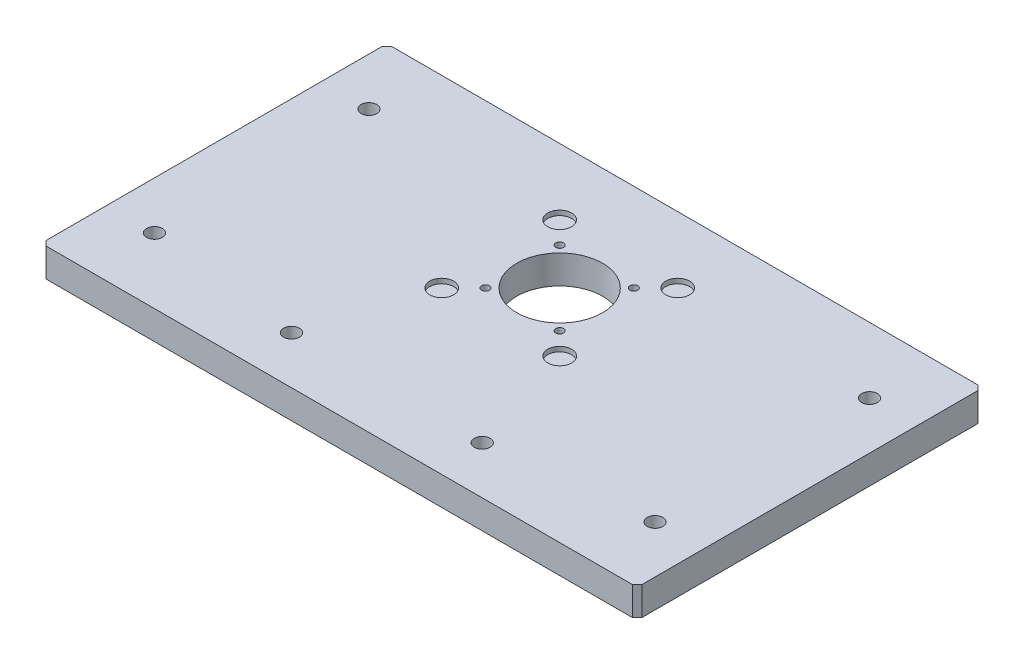
SolidWorks part; units mm, degrees
ref_plane "前视基准面" through (0, 0, 0) normal (0, 0, 1) x (1, 0, 0)
ref_plane "上视基准面" through (0, 0, 0) normal (0, 1, 0) x (1, 0, 0)
ref_plane "右视基准面" through (0, 0, 0) normal (1, 0, 0) x (0, 0, -1)
sketch "草图1" plane through (0, 0, 0) normal (0, 1, 0) x (1, 0, 0)
  line L1 (-125, -72.5) -> (125, -72.5)
  line L2 (-125, -72.5) -> (-125, 72.5)
  line L3 (-125, 72.5) -> (125, 72.5)
  line L4 (125, -72.5) -> (125, 72.5)
  line L5 (-125, -72.5) -> (125, 72.5) construction
  line L6 (-125, 72.5) -> (125, -72.5) construction
  point P0 (0, 0)
  dimension "D1" = 250
  dimension "D2" = 145
extrude "凸台-拉伸1" add sketch "草图1" along normal blind 12
chamfer "倒角1" distance 2 angle 45 4 edges at (125, 6, 72.5) (-125, 6, 72.5) (-125, 6, -72.5) (125, 6, -72.5)
sketch "草图2" plane through (0, 12, 0) normal (0, 1, 0) x (1, 0, 0)
  circle A0 centre (0, 20) radius 18
  dimension "D1" = 36
  dimension "D2" = 20
extrude "切除-拉伸1" cut sketch "草图2" against normal through all
sketch "草图5" plane through (0, 0, 0) normal (0, -1, 0) x (-1, 0, 0)
  point P0 (15.5563, 35.5563)
  point P3 (-15.5563, 35.5563)
  point P6 (-15.5563, 4.4437)
  point P9 (15.5563, 4.4437)
hole_wizard "M4 螺纹孔1" positions "草图5" profile "草图4" tap size "M4" standard "GB" end condition through all
sketch "草图4" plane through (-15.5563, 0, -35.5563) normal (1, 0, 0) x (0, 0, -1)
  line L0 (0, 0) -> (0, 12)
  line L1 (0, 12) -> (1.65, 12)
  line L2 (1.65, 12) -> (1.65, 0)
  line L5 (1.65, 0) -> (0, 0)
  line L11 (0, -6.35) -> (0, 107.95) construction
  dimension "通孔螺纹孔钻头直径" = 3.3
  dimension "通孔螺纹孔钻头深度" = 12
sketch "草图10" plane through (0, 0, 0) normal (0, -1, 0) x (-1, 0, 0)
  line L0 (0, 0) -> (0, -84.1635) construction
  line L2 (123, -72.5) -> (-123, -72.5) construction
  line L3 (-125, -70.5) -> (-125, 70.5) construction
  line L4 (125, 0) -> (-125, 0) construction
  line L5 (125, 70.5) -> (125, -70.5) construction
  point P0 (-40, -52.5)
  point P4 (-105, 45)
  point P6 (-105, -45)
  point P28 (105, 45)
  point P29 (105, -45)
  point P30 (40, -52.5)
  dimension "D1" = 80
  dimension "D2" = 20
  dimension "D3" = 20
  dimension "D4" = 90
hole_wizard "M6 六角圆柱头螺钉的柱形沉头孔1" positions "草图10" profile "草图9" counterbore size "M6" standard "GB" end condition through all
sketch "草图9" plane through (40, 0, 52.5) normal (1, 0, 0) x (0, 0, -1)
  line L0 (0, 0) -> (0, 12)
  line L1 (0, 12) -> (3.3, 12)
  line L3 (3.3, 12) -> (3.3, 6.8)
  line L4 (3.3, 6.8) -> (5.5, 6.8)
  line L5 (5.5, 6.8) -> (5.5, 0)
  line L7 (5.5, 0) -> (0, 0)
  line L11 (0, -6.35) -> (0, 107.95) construction
  dimension "通孔孔直径" = 6.6
  dimension "通孔孔深度" = 12
  dimension "柱形沉头孔直径" = 11
  dimension "柱形沉头孔深度" = 6.8
sketch "草图11" plane through (0, 12, 0) normal (0, 1, 0) x (1, 0, 0)
  circle A0 centre (24.7487, -4.7487) radius 5
  circle A1 centre (-24.7487, -4.7487) radius 5
  circle A2 centre (-24.7487, 44.7487) radius 5
  circle A3 centre (24.7487, 44.7487) radius 5
  dimension "D1" = 10
extrude "切除-拉伸2" cut sketch "草图11" against normal blind 2
